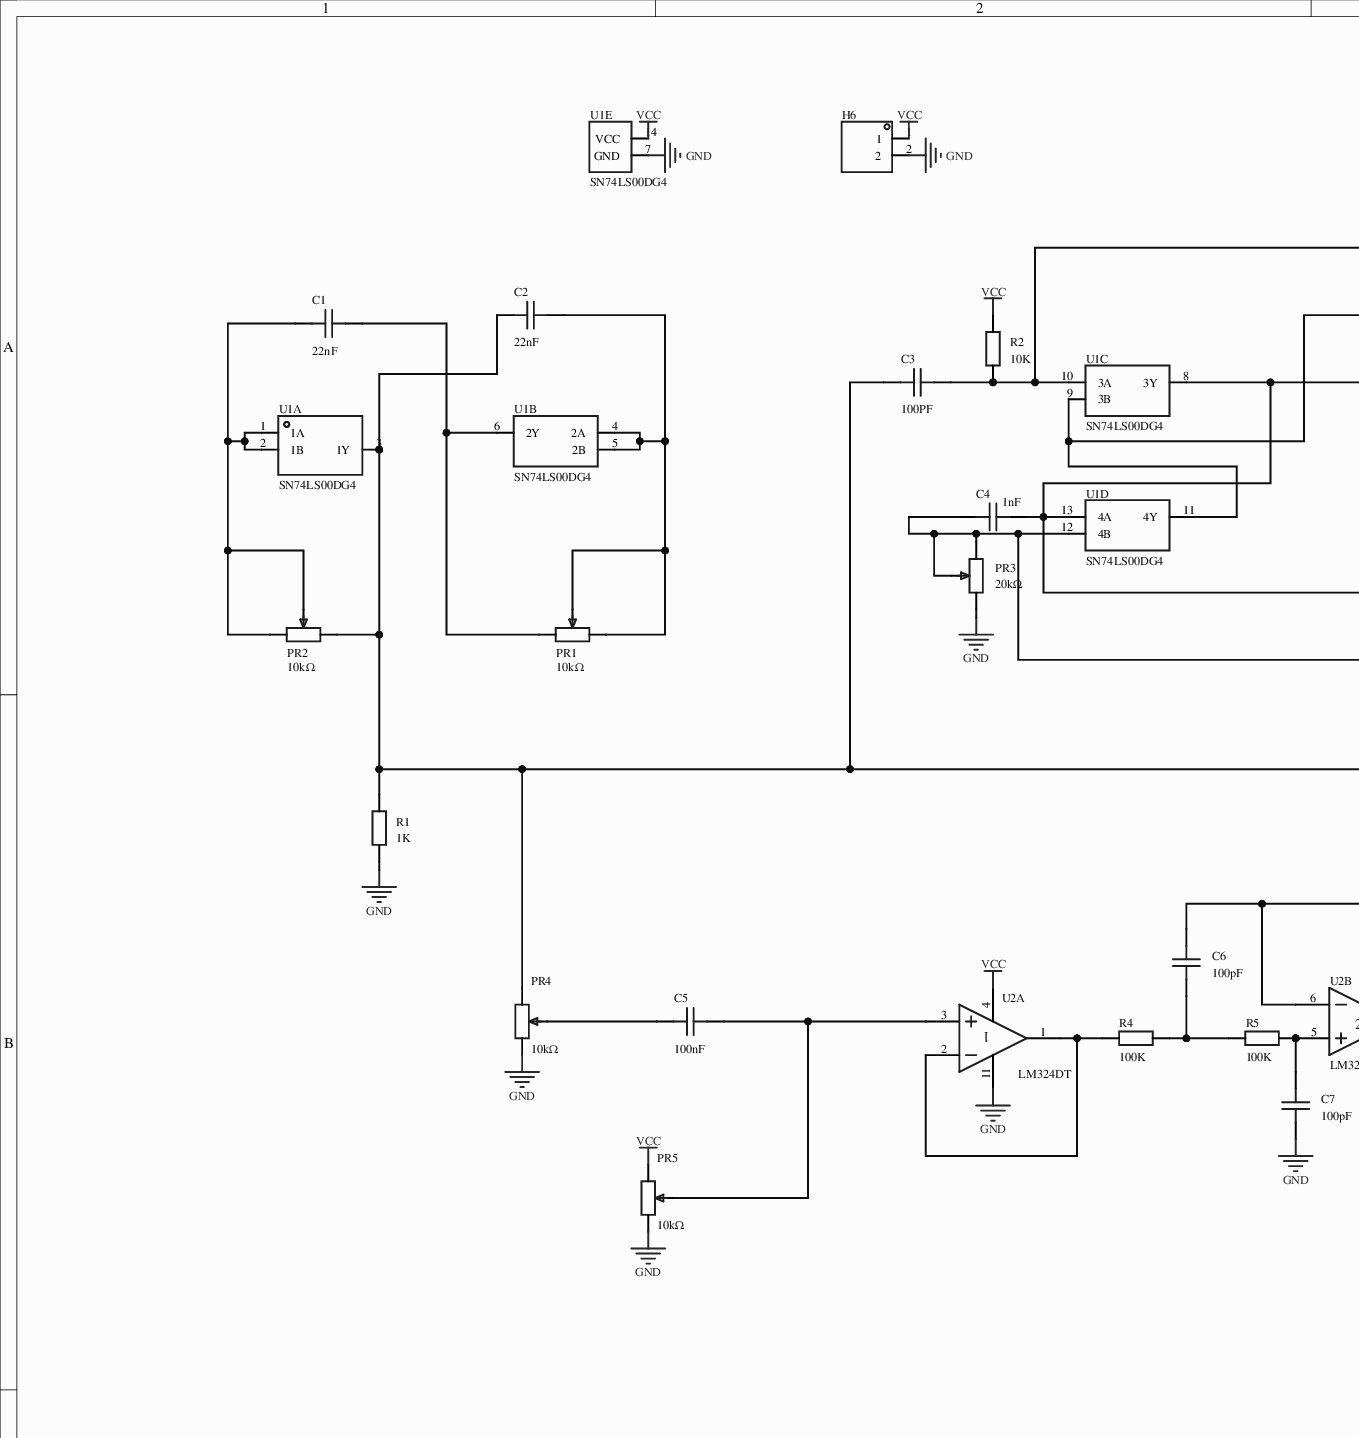
[diagram p0: MISC89095-3.schdoc, top left]
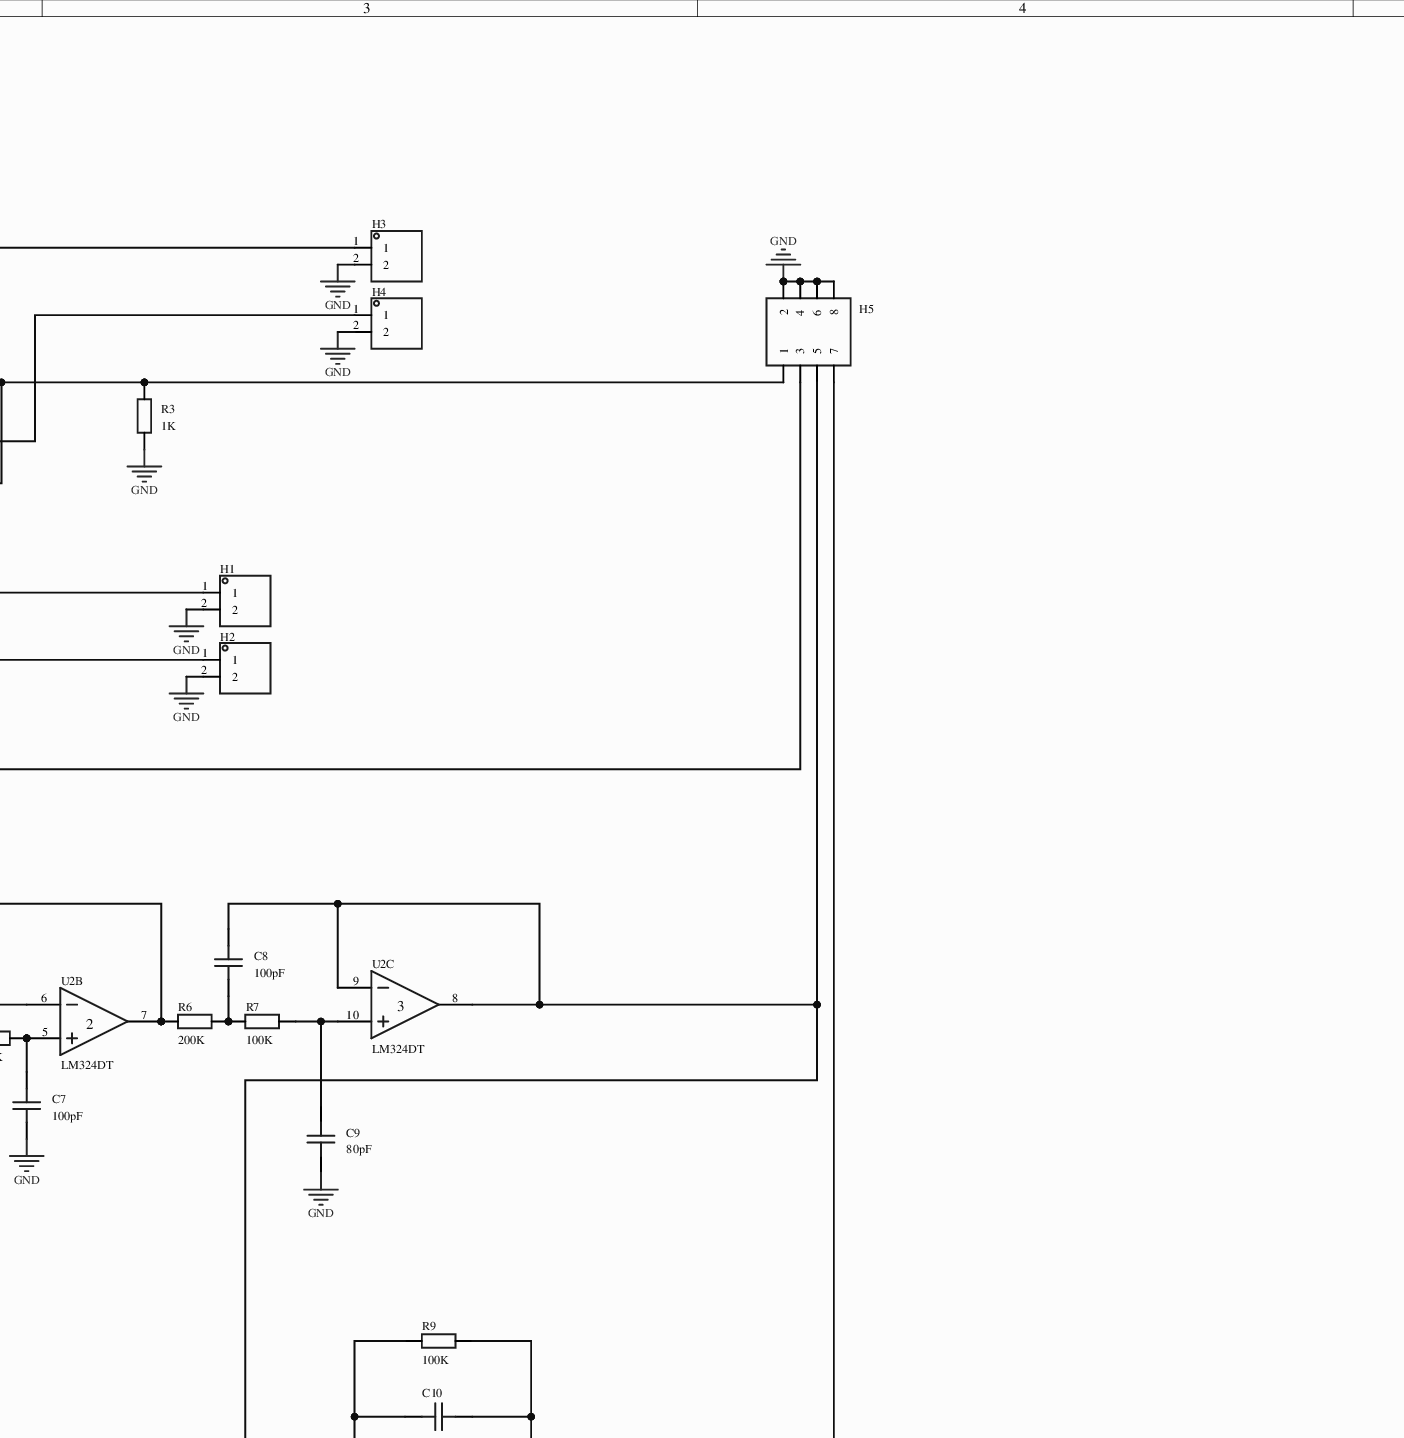
[diagram p1: MISC89095-3.schdoc, top middle]
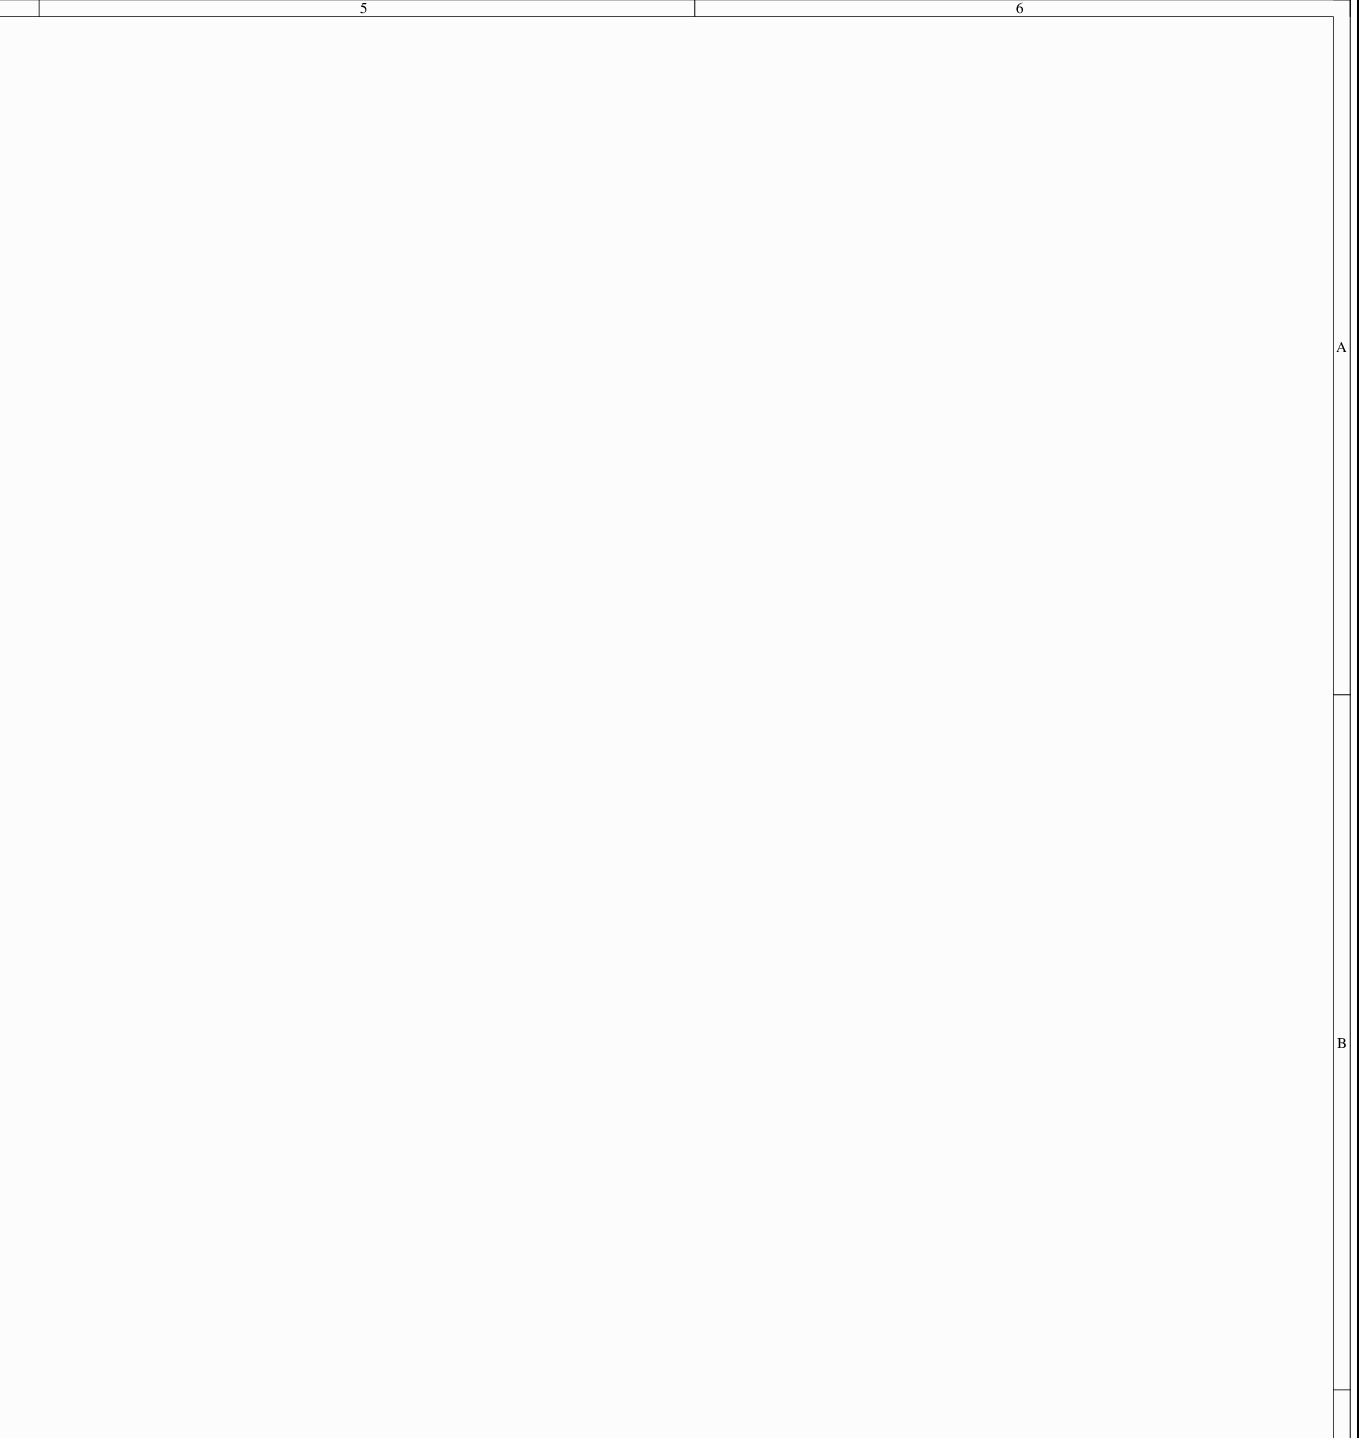
[diagram p2: MISC89095-3.schdoc, top right]
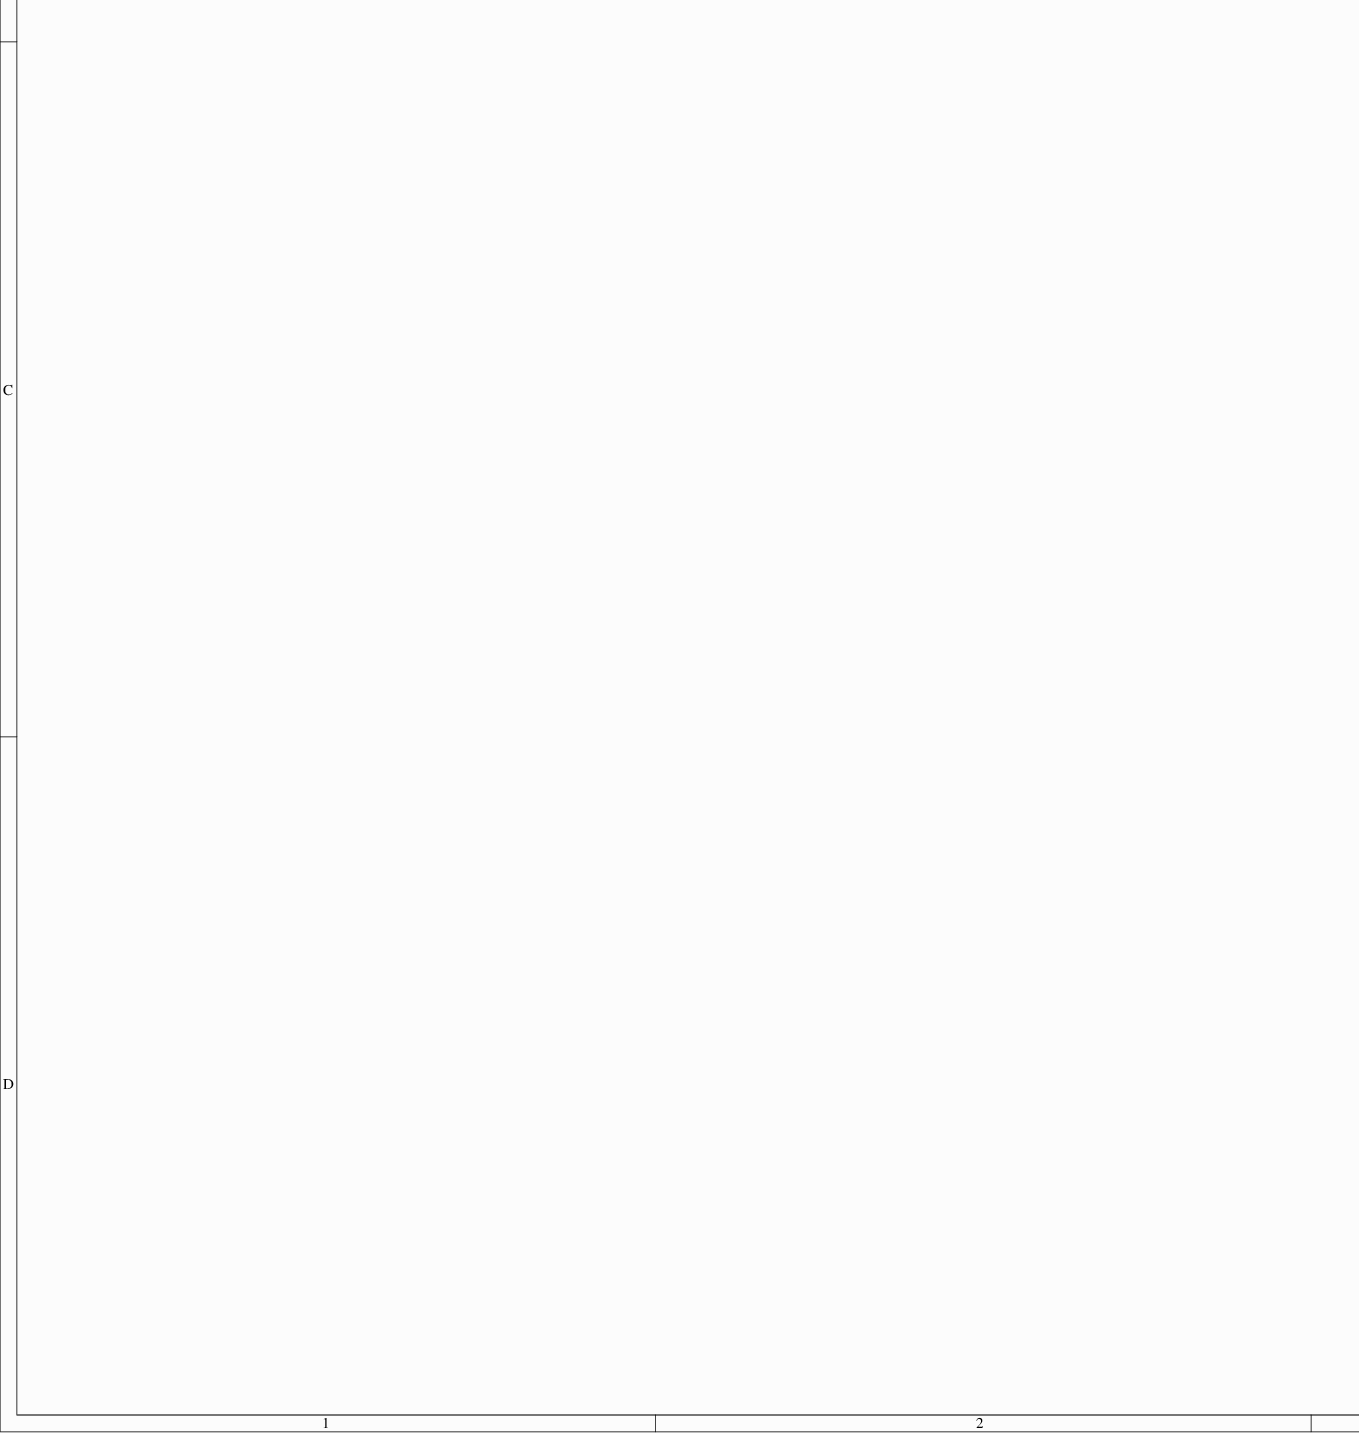
[diagram p3: MISC89095-3.schdoc, bottom left]
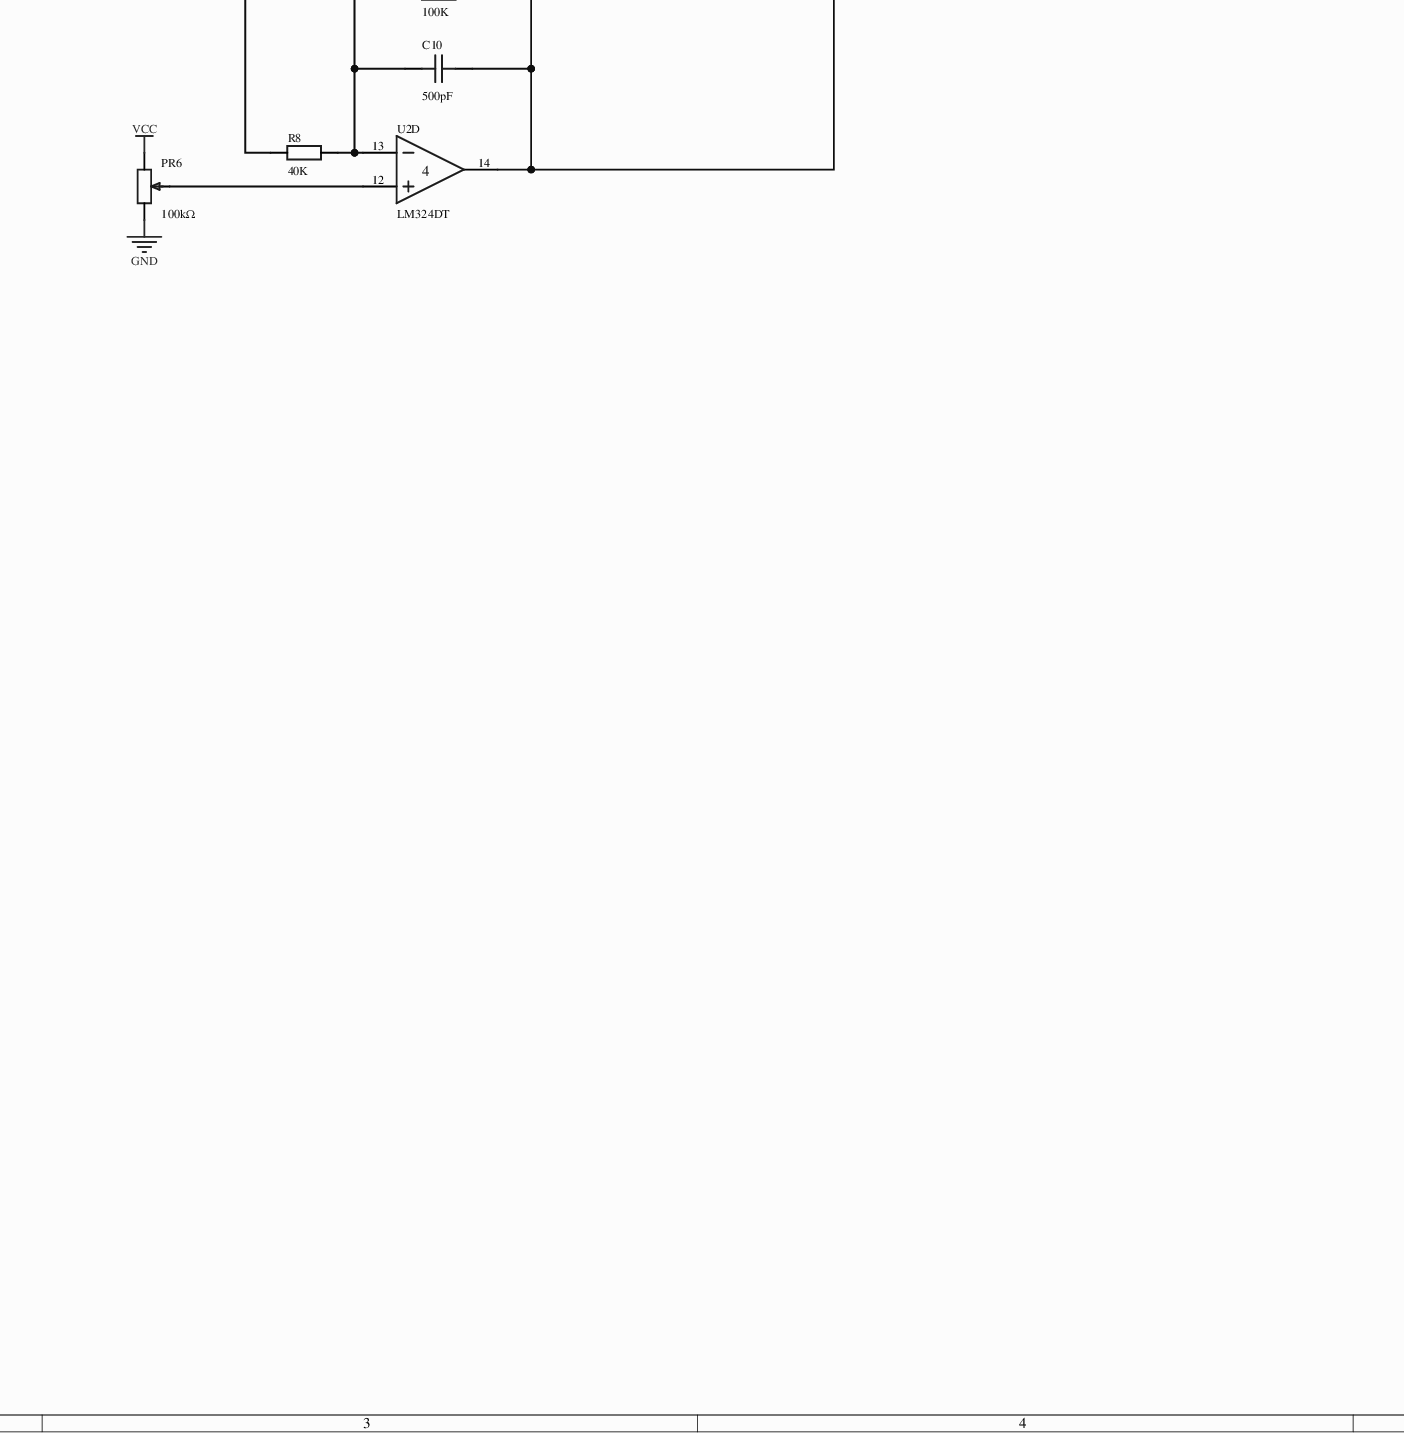
[diagram p4: MISC89095-3.schdoc, bottom middle]
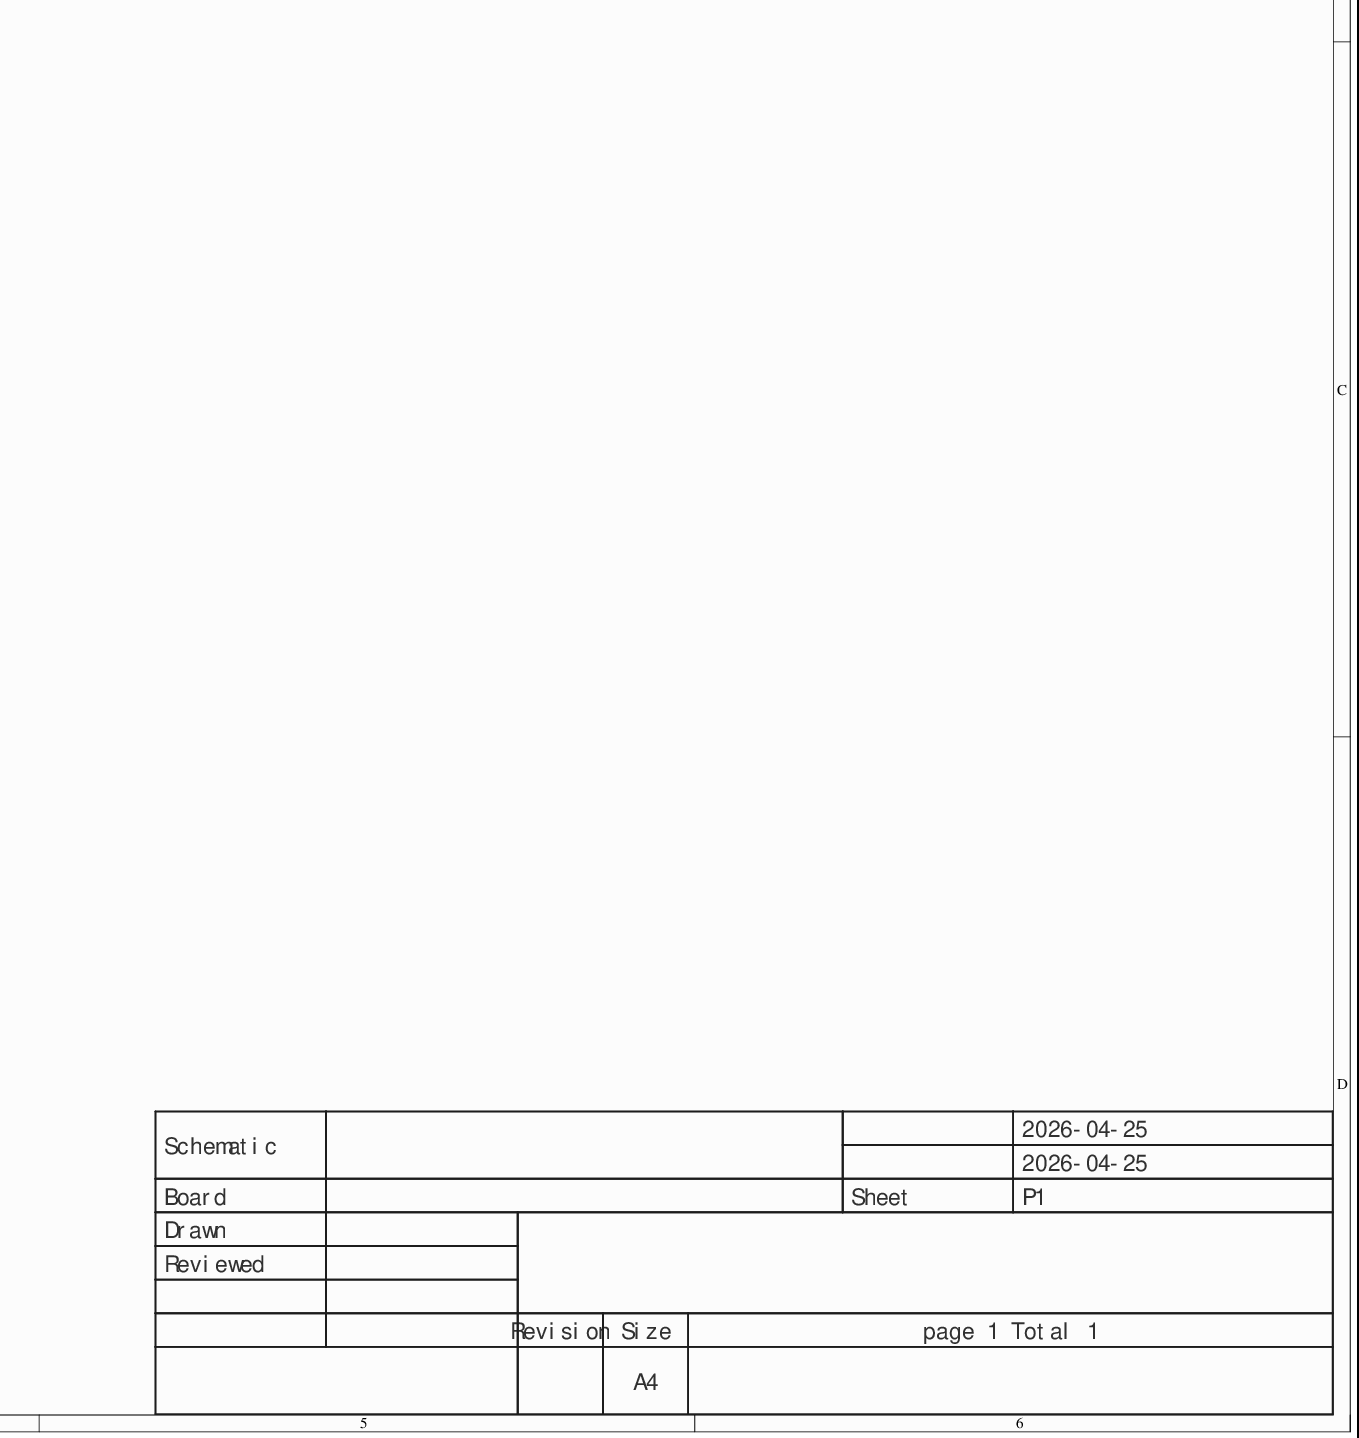
[diagram p5: MISC89095-3.schdoc, bottom right]
# Altium project MISC89095-2.PrjPcb
1 sheet, 33 parts. Net scope: global (net labels, ports and power ports of the same name join across sheets).
Board file: MISC89095.pcbdoc

## Sheet MISC89095-3.schdoc
size 594 x 419 mm; Version: V1.0; @Project Name: MISC89095; @Update Date: 2026-04-25; @Create Date: 2026-04-25; @Board Name: MISC89095; @Create Time: 10:37:37; @Page Count: 1; @Page No: 1; @Schematic Name: MISC89095; @Update Time: 10:37:37; Size: A4

### Parts
C1  22nF  [C0603]
C2  22nF  [C0603]
C3  100PF  [C0603]
C4  1nF  [C0603]
C5  100nF  [C0603]
C6  100pF  [C0603]
C7  100pF  [C0603]
C8  100pF  [C0603]
C9  80pF  [C0603]
C10  500pF  [C0603]
H1  (no value)  [HDR-TH_2P-P2.54-V-M-1]
H2  (no value)  [HDR-TH_2P-P2.54-V-M-1]
H3  (no value)  [HDR-TH_2P-P2.54-V-M-1]
H4  (no value)  [HDR-TH_2P-P2.54-V-M-1]
H5  (no value)  [HDR-TH_8P-P2.54-V-F-R2-C4-S2.54-1]
H6  (no value)  [HDR-TH_2P-P2.54-V-M-1]
PR1  10kΩ  [R_3296]
PR2  10kΩ  [R_3296]
PR3  20kΩ  [R_3296]
PR4  10kΩ  [R_3296]
PR5  10kΩ  [R_3296]
PR6  100kΩ  [R_3296]
R1  1K  [R0603]
R2  10K  [R0603]
R3  1K  [R0603]
R4  100K  [R0603]
R5  100K  [R0603]
R6  200K  [R0603]
R7  100K  [R0603]
R8  40K  [R0603]
R9  100K  [R0603]
U1  SN74LS00DG4  [SOIC-14_L8.7-W3.9-P1.27-LS6.0-BL]  (parts A,B,C,D,E of 5)
U2  LM324DT  [SOIC-14_L8.7-W3.9-P1.27-LS6.0-BL]  (parts A,B,C,D of 4)

### Nets
GND: C7.1 C9.1 H1.2 H2.2 H3.2 H4.2 H5.2 H5.4 H5.6 H5.8 H6.2 PR3.3 PR4.1 PR5.1 PR6.1 R1.1 R3.1 U1.7(GND) U2.11(VCC+)
VCC: H6.1 PR5.3 PR6.3 R2.2 U1.14(VCC) U2.4(VCC-)
NetC1_1: C1.1 PR2.2 PR2.3 U1.1(1A) U1.2(1B)
NetC1_2: C1.2 PR1.3 U1.6(2Y)
NetC2_1: C2.1 C3.1 H5.3 PR2.1 PR4.3 R1.2 U1.3(1Y)
NetC2_2: C2.2 PR1.1 PR1.2 U1.4(2A) U1.5(2B)
NetC3_2: C3.2 H3.1 R2.1 U1.10(3A)
NetC4_1: C4.1 H2.1 PR3.1 PR3.2 U1.12(4B)
NetC4_2: C4.2 H1.1 H5.1 R3.2 U1.8(3Y) U1.13(4A)
NetC5_1: C5.1 PR4.2
NetC5_2: C5.2 PR5.2 U2.3(IN1+)
NetC6_1: C6.1 R4.2 R5.1
NetC6_2: C6.2 R6.1 U2.6(IN2-) U2.7(OUT2)
NetC7_2: C7.2 R5.2 U2.5(IN2+)
NetC8_1: C8.1 R6.2 R7.1
NetC8_2: C8.2 H5.5 R8.1 U2.8(OUT3) U2.9(IN3-)
NetC9_2: C9.2 R7.2 U2.10(IN3+)
NetC10_1: C10.1 H5.7 R9.2 U2.14(OUT4)
NetC10_2: C10.2 R8.2 R9.1 U2.13(IN4-)
NetH4_1: H4.1 U1.9(3B) U1.11(4Y)
NetPR6_2: PR6.2 U2.12(IN4+)
NetR4_1: R4.1 U2.1(OUT1) U2.2(IN1-)

### Notes on the sheet
- 2026-04-25
- Schematic
- Board
- Sheet
- P1
- Drawn
- Reviewed
- Revision
- Size
- A4
- page 1 Total 1

### Library data of the parts
C1-C10 = CAP_0603: Symbol: Capacitance; ConvertToPcb: yes; ModelId: ac125912035d415993ca9572d50418b10819f05c4eef4c71ace90d822a990e87; ModelName: C0603_L1.6-W0.8-H0.8; ModelTransform: 62.992,31.496,0,0,0,0,0,0,0; Device: CAP_0603; AddInBom: yes; Supplier Footprint: 0603; FootprintName: C0603
  C1 C2: Value: 22nF
  C3: Value: 100PF
  C4: Value: 1nF
  C5: Value: 100nF
  C6-C8: Value: 100pF
  C9: Value: 80pF
  C10: Value: 500pF
H1-H4 H6 = HDR-M_2.54_1x2P: Symbol: 210S-1*2P L=11.6MMGold-plated black; ConvertToPcb: yes; ModelId: 79b2e9f2d70a4d68a1b7098f27c6d4c50819f05c4eef4c71ace90d822a990e87; ModelName: HDR-M-2.54_1x2; ModelTransform: 200,100,0,0,0,0,0,0,-118.11; Device: HDR-M_2.54_1x2P; AddInBom: yes; SupplierPart: C124375; Supplier Footprint: 插件; FootprintName: HDR-TH_2P-P2.54-V-M-1
H5 = HDR-F_2.54_2x4: Symbol: HDR-F-2.54_2x4; ConvertToPcb: yes; ModelId: 64729f32a5874cf59655d275a66f10500819f05c4eef4c71ace90d822a990e87; ModelName: HDR2.54-F-LI-2X4P; ModelTransform: 399.999,200,0,0,0,0,0,0,-118.11; Device: HDR-F_2.54_2x4; AddInBom: yes; SupplierPart: C92271; Supplier Footprint: 插件; FootprintName: HDR-TH_8P-P2.54-V-F-R2-C4-S2.54-1
PR1-PR6 = R_3296: ConvertToPcb: yes; ModelId: b182808559bb43bda9e7de64b64134cb0819f05c4eef4c71ace90d822a990e87; ModelName: 3296W; ModelTransform: 373.98,188.96,590.49,180,0,0,0,0,-140; Symbol: R_3296; Device: R_3296; AddInBom: yes; Supplier Footprint: 直插; FootprintName: R_3296
  PR1 PR2 PR4 PR5: Value: 10kΩ
  PR3: Value: 20kΩ
  PR6: Value: 100kΩ
R1-R9 = Res_0603: Symbol: Resistor; ConvertToPcb: yes; ModelId: fc143cca1e79419f9cd78b61e9279f080819f05c4eef4c71ace90d822a990e87; ModelTransform: 31.8897,63.7794,0,90,0,0,0,0,0; Device: Res_0603; AddInBom: yes; Supplier Footprint: 0603; FootprintName: R0603; ModelName: R0603
  R1 R3: Value: 1K
  R2: Value: 10K
  R4 R5 R7 R9: Value: 100K
  R6: Value: 200K
  R8: Value: 40K
U1 = SN74LS00DG4: Manufacturer: TI(德州仪器); Add into BOM: yes; 3D Model: 8dbf5b715d42428c85558507ae5a252b0819f05c4eef4c71ace90d822a990e87; 3D Model Transform: 338.583,236.22,0,0,0,0,0,0.001,0; ModelName: SOIC-14_L8.6-W3.9-H1.8-LS6.0-P1.27; Symbol: SN74LS00DG4; Device: SN74LS00DG4; Convert to PCB: yes; LCSC Part Name: SN74LS00DG4; Supplier Part: C4470704; Manufacturer Part: SN74LS00DG4; Supplier Footprint: SOIC-14; JLCPCB Part Class: Extended Part; Datasheet: https://www.ti.com/cn/lit/gpn/sn74ls00; Supplier: LCSC; FootprintName: SOIC-14_L8.7-W3.9-P1.27-LS6.0-BL
U2 = LM324DT: 放大器数:4;轨到轨:-;增益带宽积(GBW):1.3MHz;输入失调电压(Vos):5mV;压摆率(SR):400V/ms;输入偏置电流(Ib):300nA;; Manufacturer: ST(意法半导体); Relevance: []; AddInBom: yes; ModelId: 8dbf5b715d42428c85558507ae5a252b0819f05c4eef4c71ace90d822a990e87; ModelName: SOIC-14_L8.6-W3.9-H1.8-LS6.0-P1.27; ModelTransform: 338.583,236.22,0,0,0,0,0,0.001,0; Number of Channels: 4; Maximum Power Supply Range (Vdd-Vss): 30V; Gain Bandwidth Product: 1.3MHz; Vos - Input Offset Voltage: 5mV; Input Offset Voltage Drift(Vos TC): 30uV/℃; Ib - Input Bias Current: 300nA; Input Offset Current(Ios): 20nA; Input Voltage Noise Density: 40nV/√Hz@1kHz; Common Mode Rejection Ratio(CMRR): 80dB; Input offset current drift(Ios TC): 200pA/℃; Quiescent Current: 1.2mA; Output Current: 70mA; Single supply: 3V~30V; Dual Supply: -15V~-1.5V; 1.5V~15V; Description: Amplifiers: 4; rail-to-rail: -; gain-bandwidth product (GBW): 1.3MHz; input offset voltage (Vos): 5mV; slew rate (SR): 400V/ms; input bias current (Ib): 300nA;; Symbol: LM324DT; Device: LM324DT; LCSC Part Name: 低功耗四路运算放大器; SupplierPart: C71035; ManufacturerPart: LM324DT; Supplier Footprint: SOIC-14; JLCPCB Part Class: Basic Part; Datasheet: https://item.szlcsc.com/datasheet/LM324DT/72134.html; Supplier: LCSC; ConvertToPcb: yes; FootprintName: SOIC-14_L8.7-W3.9-P1.27-LS6.0-BL; Rail to Rail: -; Slew Rate: 400V/ms; Operating Temperature: 0℃~+70℃; Features: Internal compensation